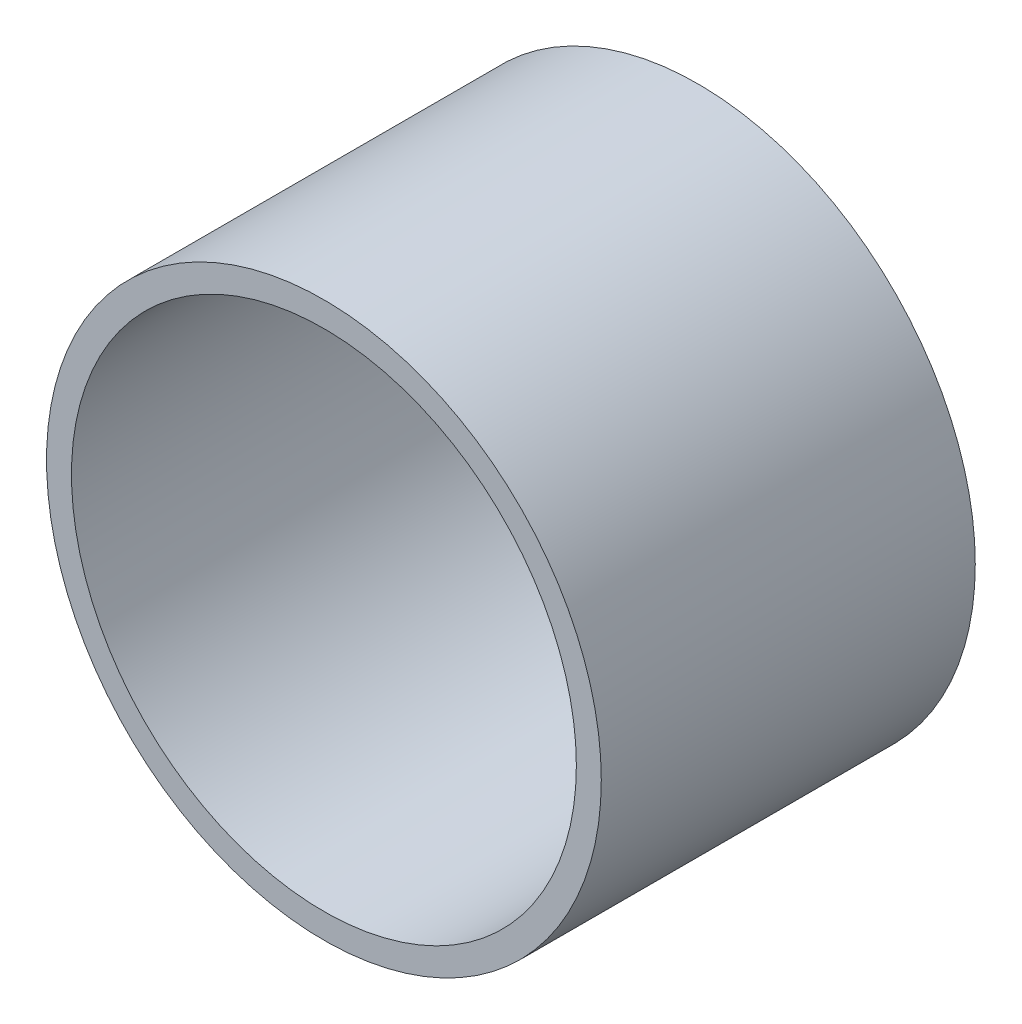
from build123d import *

# Parameters (mm, degrees)
SKETCH1_R           = 44.5
SKETCH1_R_2         = 40.5
BOSS_EXTRUDE1_DEPTH = 60


with BuildPart() as part:
    # Sketch1 → Boss-Extrude1 (new body)
    with BuildSketch(Plane.XY):
        with Locations((-1060, 0)):
            Circle(SKETCH1_R)
        with Locations((-1060, 0)):
            Circle(SKETCH1_R_2, mode=Mode.SUBTRACT)
    extrude(amount=BOSS_EXTRUDE1_DEPTH)


solid = part.part
